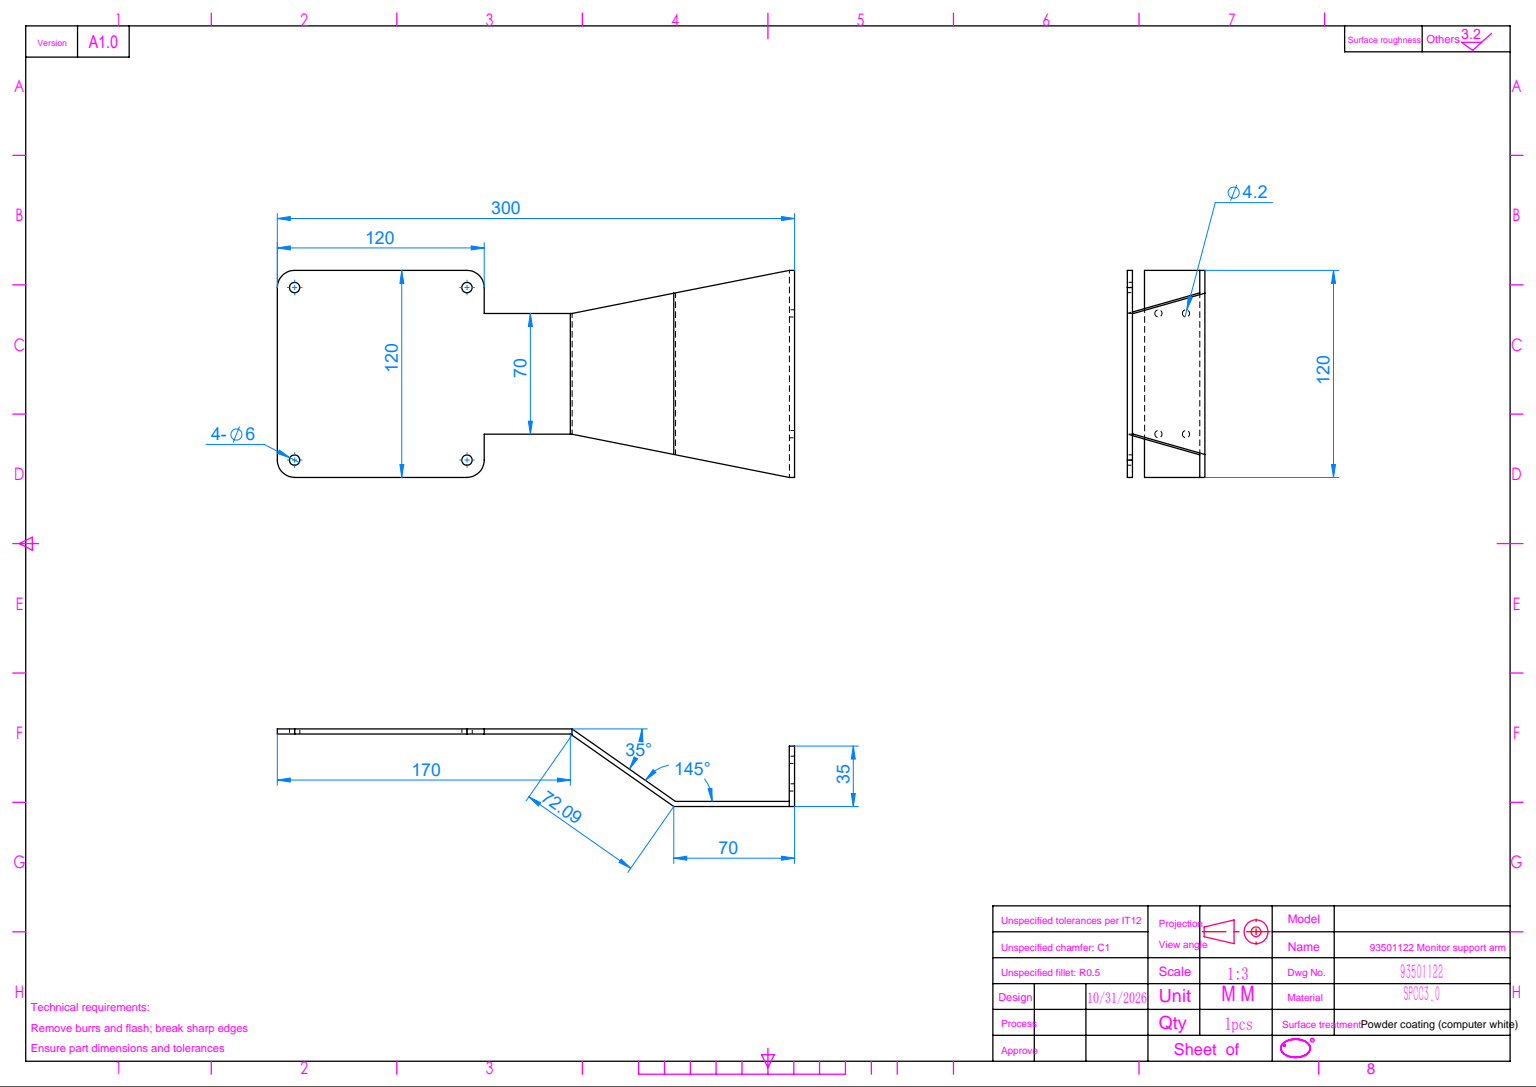
from build123d import *

# Parameters (mm, degrees)
EXTRUDE_1_DEPTH      = 60
EXTRUDE_1_DEPTH_BACK = 60
CUT_EXTRUDE_1_DEPTH  = 310.232921921
FILLET_1_R           = 10
CUT_EXTRUDE_2_REACH  = 311.233
SKETCH_3_R           = 3
CUT_EXTRUDE_3_REACH  = 310.811
SKETCH_4_R           = 2.1


with BuildPart() as part:
    # 草图1 → 拉伸-薄壁1 (new, two sides: drawn at the far end of the back side and taken through both)
    with BuildSketch(Plane.XY.offset(-EXTRUDE_1_DEPTH_BACK)):
        Polygon((0, 0), (170, 0), (230, -42), (300, -42), (300, -7), (297, -7), (297, -39), (230.945666692, -39), (170.945666692, 3), (0, 3), align=None)
    extrude(amount=EXTRUDE_1_DEPTH + EXTRUDE_1_DEPTH_BACK)

    # 草图2 → 切除-拉伸1 (cut, through all)
    with BuildSketch(Plane(origin=(0, 3, 0), x_dir=(1, 0, 0), z_dir=(0, 1, 0))):
        Polygon((120, 60), (120, 35), (170.945666692, 35), (297, 60), align=None)
        Polygon((297, -60), (120, -60), (120, -35), (170.945666692, -35), align=None)
    extrude(amount=-CUT_EXTRUDE_1_DEPTH, mode=Mode.SUBTRACT)

    # 圆角1
    fillet_1_edges = [part.edges().sort_by_distance(p)[0] for p in [
        (0, 1.5, -60),
        (0, 1.5, 60),
        (120, 1.5, -60),
        (120, 1.5, 60),
    ]]
    fillet(fillet_1_edges, radius=FILLET_1_R)

    # 草图3 → 切除-拉伸2 (cut, up to next)
    with BuildSketch(Plane(origin=(0, 3, 0), x_dir=(1, 0, 0), z_dir=(0, 1, 0)), mode=Mode.PRIVATE) as cut_extrude_2_sk1:
        with Locations(Location((10, 50, 0), (0, 0, 270))):
            Circle(SKETCH_3_R)
    cut_extrude_2_tool1 = extrude(cut_extrude_2_sk1.sketch, amount=-CUT_EXTRUDE_2_REACH, mode=Mode.PRIVATE) & part.part
    # 草图3 → 切除-拉伸2 (cut, up to next)
    with BuildSketch(Plane(origin=(0, 3, 0), x_dir=(1, 0, 0), z_dir=(0, 1, 0)), mode=Mode.PRIVATE) as cut_extrude_2_sk2:
        with Locations(Location((110, 50, 0), (0, 0, 270))):
            Circle(SKETCH_3_R)
    cut_extrude_2_tool2 = extrude(cut_extrude_2_sk2.sketch, amount=-CUT_EXTRUDE_2_REACH, mode=Mode.PRIVATE) & part.part
    # 草图3 → 切除-拉伸2 (cut, up to next)
    with BuildSketch(Plane(origin=(0, 3, 0), x_dir=(1, 0, 0), z_dir=(0, 1, 0)), mode=Mode.PRIVATE) as cut_extrude_2_sk3:
        with Locations(Location((110, -50, 0), (0, 0, 270))):
            Circle(SKETCH_3_R)
    cut_extrude_2_tool3 = extrude(cut_extrude_2_sk3.sketch, amount=-CUT_EXTRUDE_2_REACH, mode=Mode.PRIVATE) & part.part
    # 草图3 → 切除-拉伸2 (cut, up to next)
    with BuildSketch(Plane(origin=(0, 3, 0), x_dir=(1, 0, 0), z_dir=(0, 1, 0)), mode=Mode.PRIVATE) as cut_extrude_2_sk4:
        with Locations(Location((10, -50, 0), (0, 0, 270))):
            Circle(SKETCH_3_R)
    cut_extrude_2_tool4 = extrude(cut_extrude_2_sk4.sketch, amount=-CUT_EXTRUDE_2_REACH, mode=Mode.PRIVATE) & part.part
    add(cut_extrude_2_tool1.solids().sort_by_distance((10, 3, -50))[0], mode=Mode.SUBTRACT)
    add(cut_extrude_2_tool2.solids().sort_by_distance((110, 3, -50))[0], mode=Mode.SUBTRACT)
    add(cut_extrude_2_tool3.solids().sort_by_distance((110, 3, 50))[0], mode=Mode.SUBTRACT)
    add(cut_extrude_2_tool4.solids().sort_by_distance((10, 3, 50))[0], mode=Mode.SUBTRACT)

    # 草图4 → 切除-拉伸3 (cut, up to next)
    with BuildSketch(Plane(origin=(300, 0, 0), x_dir=(0, 0, -1), z_dir=(1, 0, 0)), mode=Mode.PRIVATE) as cut_extrude_3_sk1:
        with Locations(Location((-35, -15, 0), (0, 0, 90))):
            Circle(SKETCH_4_R)
    cut_extrude_3_tool1 = extrude(cut_extrude_3_sk1.sketch, amount=-CUT_EXTRUDE_3_REACH, mode=Mode.PRIVATE) & part.part
    # 草图4 → 切除-拉伸3 (cut, up to next)
    with BuildSketch(Plane(origin=(300, 0, 0), x_dir=(0, 0, -1), z_dir=(1, 0, 0)), mode=Mode.PRIVATE) as cut_extrude_3_sk2:
        with Locations(Location((-35, -31, 0), (0, 0, 90))):
            Circle(SKETCH_4_R)
    cut_extrude_3_tool2 = extrude(cut_extrude_3_sk2.sketch, amount=-CUT_EXTRUDE_3_REACH, mode=Mode.PRIVATE) & part.part
    # 草图4 → 切除-拉伸3 (cut, up to next)
    with BuildSketch(Plane(origin=(300, 0, 0), x_dir=(0, 0, -1), z_dir=(1, 0, 0)), mode=Mode.PRIVATE) as cut_extrude_3_sk3:
        with Locations(Location((35, -31, 0), (0, 0, 90))):
            Circle(SKETCH_4_R)
    cut_extrude_3_tool3 = extrude(cut_extrude_3_sk3.sketch, amount=-CUT_EXTRUDE_3_REACH, mode=Mode.PRIVATE) & part.part
    # 草图4 → 切除-拉伸3 (cut, up to next)
    with BuildSketch(Plane(origin=(300, 0, 0), x_dir=(0, 0, -1), z_dir=(1, 0, 0)), mode=Mode.PRIVATE) as cut_extrude_3_sk4:
        with Locations(Location((35, -15, 0), (0, 0, 90))):
            Circle(SKETCH_4_R)
    cut_extrude_3_tool4 = extrude(cut_extrude_3_sk4.sketch, amount=-CUT_EXTRUDE_3_REACH, mode=Mode.PRIVATE) & part.part
    add(cut_extrude_3_tool1.solids().sort_by_distance((300, -15, 35))[0], mode=Mode.SUBTRACT)
    add(cut_extrude_3_tool2.solids().sort_by_distance((300, -31, 35))[0], mode=Mode.SUBTRACT)
    add(cut_extrude_3_tool3.solids().sort_by_distance((300, -31, -35))[0], mode=Mode.SUBTRACT)
    add(cut_extrude_3_tool4.solids().sort_by_distance((300, -15, -35))[0], mode=Mode.SUBTRACT)


solid = part.part
